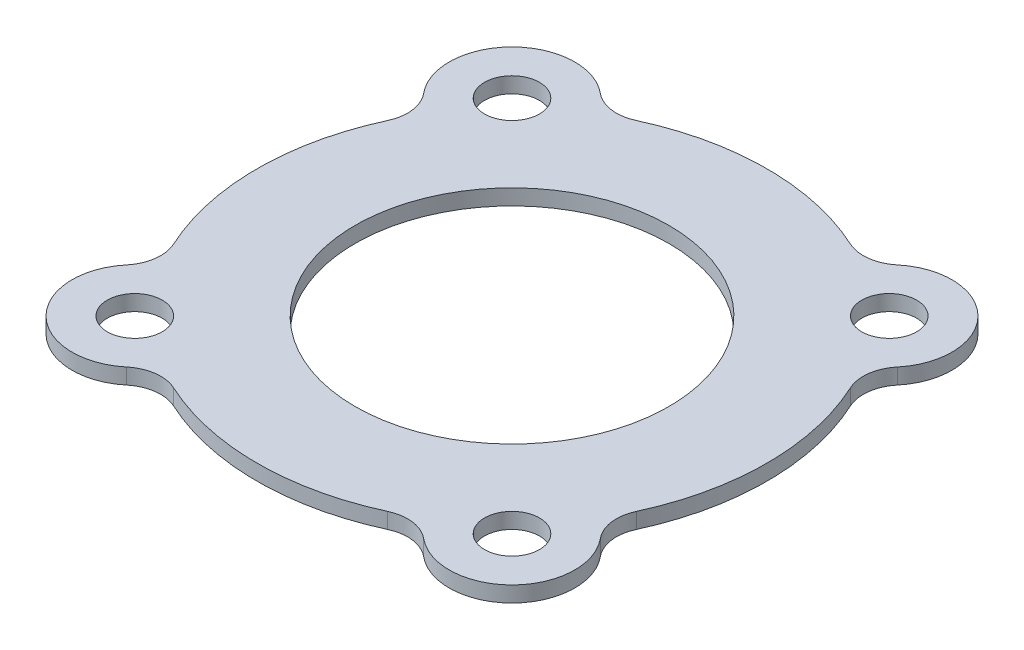
SolidWorks part; units mm, degrees
ref_plane "Front Plane" through (0, 0, 0) normal (0, 0, 1) x (1, 0, 0)
ref_plane "Top Plane" through (0, 0, 0) normal (0, 1, 0) x (1, 0, 0)
ref_plane "Right Plane" through (0, 0, 0) normal (1, 0, 0) x (0, 0, -1)
other "Configuration Table"
sketch "Sketch2" plane through (0, 0, 0) normal (0, 1, 0) x (1, 0, 0)
  line L0 (0, 0) -> (-42.4288, 42.4288) construction
  line L1 (0, 0) -> (0, 52.7766) construction
  circle A0 centre (0, 0) radius 20
  arc A1 (-27.7333, 16.9444) -> (-27.7333, -16.9444) centre (0, 0) ccw
  circle A2 centre (0, 0) radius 34 construction
  arc A3 (-16.9444, 27.7333) -> (-27.7333, 16.9444) centre (-24.0416, 24.0416) ccw
  arc A4 (27.7333, 16.9444) -> (16.9444, 27.7333) centre (24.0416, 24.0416) ccw
  arc A5 (16.9444, -27.7333) -> (27.7333, -16.9444) centre (24.0416, -24.0416) ccw
  arc A6 (-27.7333, -16.9444) -> (-16.9444, -27.7333) centre (-24.0416, -24.0416) ccw
  arc A7 (16.9444, 27.7333) -> (-16.9444, 27.7333) centre (0, 0) ccw
  arc A8 (27.7333, -16.9444) -> (27.7333, 16.9444) centre (0, 0) ccw
  arc A9 (-16.9444, -27.7333) -> (16.9444, -27.7333) centre (0, 0) ccw
  circle A10 centre (-24.0416, 24.0416) radius 3.5
  circle A11 centre (24.0416, 24.0416) radius 3.5
  circle A12 centre (24.0416, -24.0416) radius 3.5
  circle A13 centre (-24.0416, -24.0416) radius 3.5
  point P18 (0, 0)
  point P29 (0, 0)
  dimension "D1" = 65
  dimension "D2" = 40
  dimension "D3" = 68
  dimension "D5" = 16
  dimension "D7" = 7
  dimension "D4" = 45
  dimension "D6" = 4
  dimension "D8" = 4
extrude "Boss-Extrude1" add sketch "Sketch2" along normal blind 2
fillet "Fillet1" radius 5 7 edges at (-27.7333, 1, -16.9444) (16.9444, 1, -27.7333) (27.7333, 1, -16.9444) (27.7333, 1, 16.9444) (16.9444, 1, 27.7333) (-16.9444, 1, 27.7333) (-27.7333, 1, 16.9444)
fillet "Fillet2" radius 5 1 edges at (-16.9444, 1, -27.7333)
